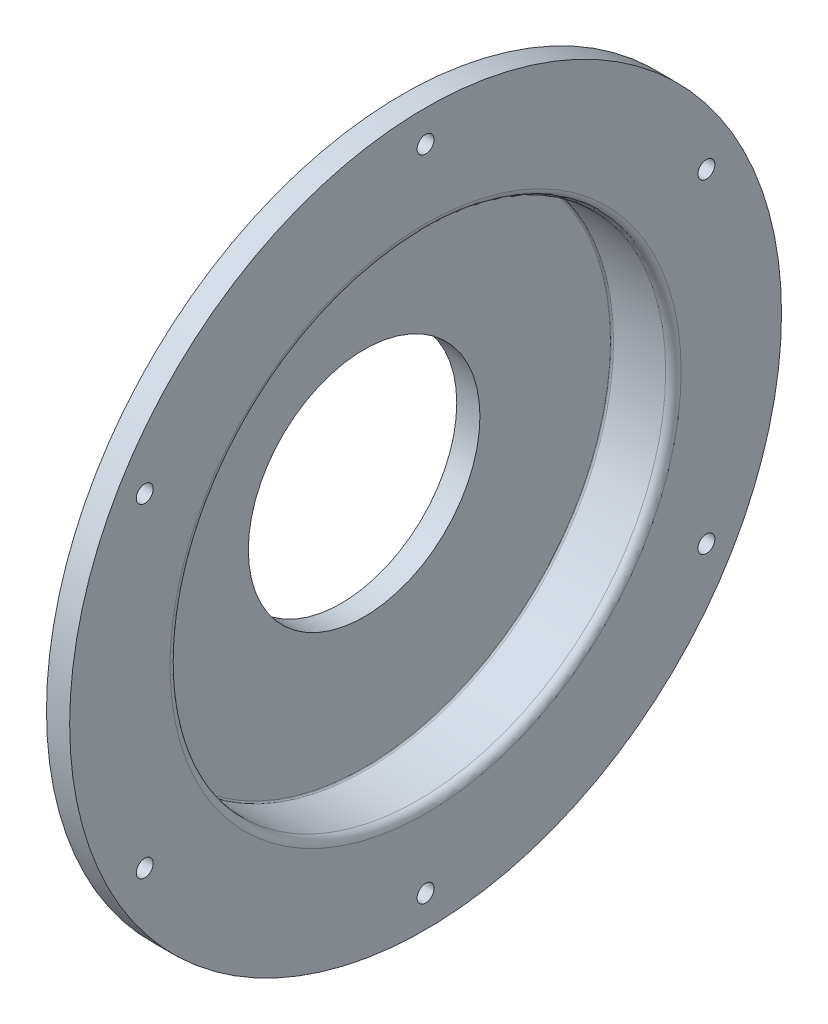
SolidWorks part; units mm, degrees
ref_plane "Front Plane" through (0, 0, 0) normal (0, 0, 1) x (1, 0, 0)
ref_plane "Top Plane" through (0, 0, 0) normal (0, 1, 0) x (1, 0, 0)
ref_plane "Right Plane" through (0, 0, 0) normal (1, 0, 0) x (0, 0, -1)
other "Configuration Table"
sketch "Sketch1" plane through (0, 0, 0) normal (0, 0, 1) x (1, 0, 0)
  line L0 (-357.6443, 160.5) -> (-391.4443, 160.5)
  line L1 (-372.6443, 175.5) -> (-402.4443, 175.5)
  line L2 (-352.6443, 230.5) -> (-352.6443, 205.5)
  line L3 (-352.6443, 205.5) -> (-352.6443, 165.5)
  line L4 (-367.6443, 230.5) -> (-367.6443, 205)
  line L5 (-367.6443, 205) -> (-367.6443, 180.5)
  line L6 (-392.4443, 159.5) -> (-392.4443, 131)
  line L7 (-392.4443, 131) -> (-392.4443, 75)
  line L8 (-407.4443, 170.5) -> (-407.4443, 131)
  line L9 (-407.4443, 131) -> (-407.4443, 75)
  line L10 (-352.6443, 230.5) -> (-367.6443, 230.5)
  line L11 (0, 0) -> (-318.2904, 0) construction
  line L12 (-55, 230.5) -> (-322.6443, 230.5) construction
  line L13 (-392.4443, 75) -> (-407.4443, 75)
  arc A0 (-357.6443, 160.5) -> (-352.6443, 165.5) centre (-357.6443, 165.5) ccw
  arc A1 (-372.6443, 175.5) -> (-367.6443, 180.5) centre (-372.6443, 180.5) ccw
  arc A2 (-391.4443, 160.5) -> (-392.4443, 159.5) centre (-391.4443, 159.5) ccw
  arc A3 (-402.4443, 175.5) -> (-407.4443, 170.5) centre (-402.4443, 170.5) ccw
revolve "Revolve1" add sketch "Sketch1" angle 360 about L11
sketch "Sketch2" plane through (-367.6443, 0, 0) normal (-1, 0, 0) x (0, 0, 1)
  circle A0 centre (0, 210) radius 5.5
  circle A1 centre (181.8653, 105) radius 5.5
  circle A2 centre (181.8653, -105) radius 5.5
  circle A3 centre (0, -210) radius 5.5
  circle A4 centre (-181.8653, -105) radius 5.5
  circle A5 centre (-181.8653, 105) radius 5.5
  point P15 (0, 0)
  dimension "D1" = 6
extrude "Cut-Extrude1" cut sketch "Sketch2" against normal blind 85
